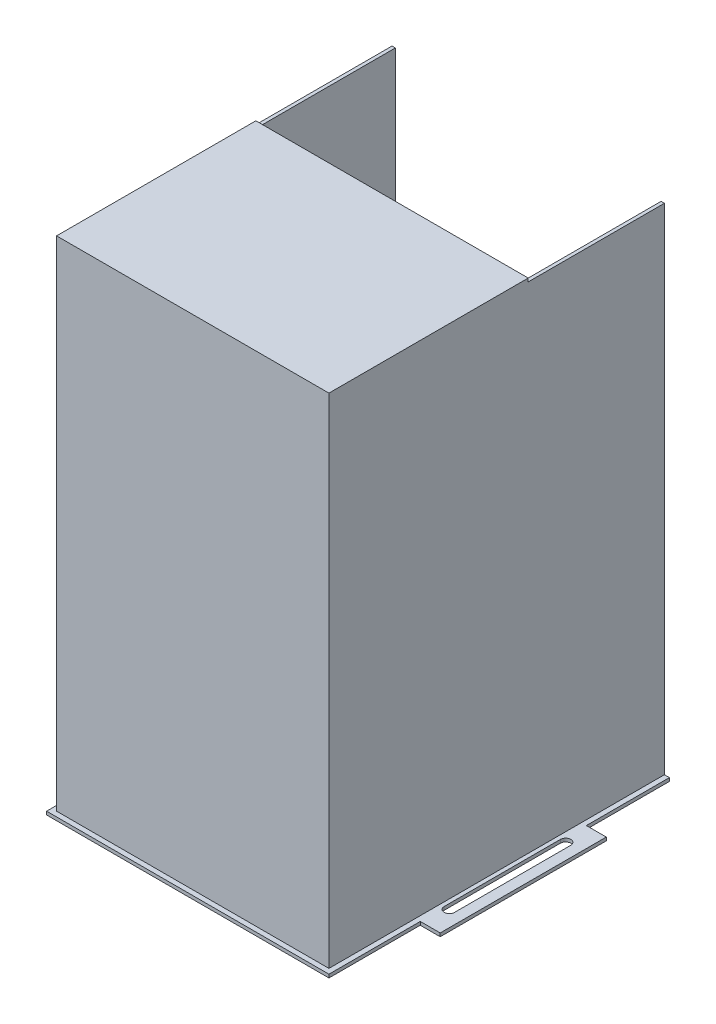
from build123d import *

# Parameters (mm, degrees)
BOSS_EXTRUDE1_DEPTH     = 300
SKETCH4_W               = 15
SKETCH4_H               = 100
BOSS_EXTRUDE3_DEPTH     = 2
CUT_EXTRUDE2_DEPTH      = 402.657814564
CUT_EXTRUDE2_DEPTH_BACK = 402.657814564
SKETCH6_W               = 164
SKETCH6_H               = 120
BOSS_EXTRUDE4_DEPTH     = 2
BOSS_EXTRUDE5_DEPTH     = 2


with BuildPart() as part:
    # Sketch1 → Boss-Extrude1 (new body)
    with BuildSketch(Plane(origin=(0, 0, 0), x_dir=(1, 0, 0), z_dir=(0, 1, 0))):
        Polygon((160, 0), (160, 200), (162, 200), (162, -2), (-2, -2), (-2, 200), (0, 200), (0, 0), align=None)
    extrude(amount=BOSS_EXTRUDE1_DEPTH)

    # Sketch4 → Boss-Extrude3 (add)
    with BuildSketch(Plane.XZ):
        with Locations((-9.5, -100)):
            Rectangle(SKETCH4_W, SKETCH4_H)
        with Locations((169.5, -100)):
            Rectangle(SKETCH4_W, SKETCH4_H)
    extrude(amount=-BOSS_EXTRUDE3_DEPTH)

    # Sketch5 → Cut-Extrude2 (cut, two sides: drawn at the far end of the back side and taken through both)
    with BuildSketch(Plane.XZ.offset(-CUT_EXTRUDE2_DEPTH_BACK)):
        with BuildLine():
            Line((-4.4, -65), (-4.4, -135))
            ThreePointArc((-4.4, -135), (-7.5, -138.1), (-10.6, -135))
            Line((-10.6, -135), (-10.6, -65))
            ThreePointArc((-10.6, -65), (-7.5, -61.9), (-4.4, -65))
        make_face()
        with BuildLine():
            Line((170.6, -65), (170.6, -135))
            ThreePointArc((170.6, -135), (167.5, -138.1), (164.4, -135))
            Line((164.4, -135), (164.4, -65))
            ThreePointArc((164.4, -65), (167.5, -61.9), (170.6, -65))
        make_face()
    extrude(amount=CUT_EXTRUDE2_DEPTH + CUT_EXTRUDE2_DEPTH_BACK, mode=Mode.SUBTRACT)

    # Sketch6 → Boss-Extrude4 (add)
    with BuildSketch(Plane(origin=(0, 300, 0), x_dir=(1, 0, 0), z_dir=(0, 1, 0))):
        with Locations((80, 58)):
            Rectangle(SKETCH6_W, SKETCH6_H)
    extrude(amount=BOSS_EXTRUDE4_DEPTH)

    # Sketch7 → Boss-Extrude5 (add)
    with BuildSketch(Plane.XZ):
        Polygon((-2, -200), (-2, 2), (162, 2), (162, -200), (165, -200), (165, -137.966768061), (163.387303915, -137.966768061), (163.387303915, -56.304675841), (165, -56.304675841), (165, 5), (-5, 5), (-5, -59.253655593), (-3.5, -59.253655593), (-3.5, -137.966768061), (-5, -137.966768061), (-5, -200), align=None)
    extrude(amount=-BOSS_EXTRUDE5_DEPTH)


solid = part.part
